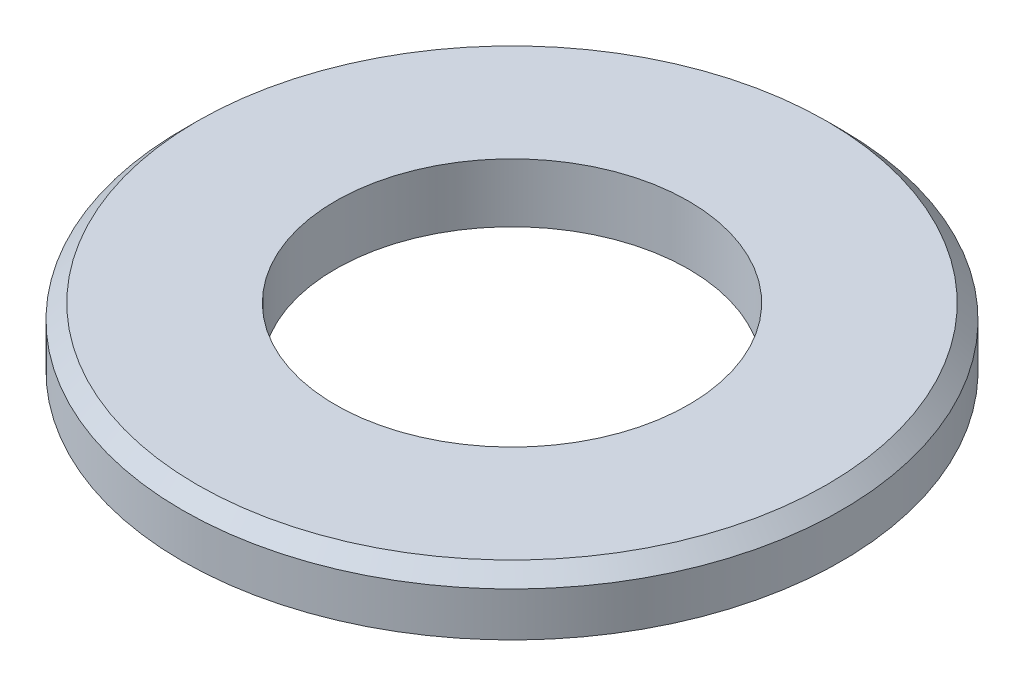
SolidWorks part; units mm, degrees
material "钢"
ref_plane "Plane1" through (0, 0, 0) normal (0, 0, 1) x (1, 0, 0)
ref_plane "Plane2" through (0, 0, 0) normal (0, 1, 0) x (1, 0, 0)
ref_plane "Plane3" through (0, 0, 0) normal (1, 0, 0) x (0, 0, -1)
sketch "Dimension sketch" plane through (0, 0, 0) normal (0, 0, 1) x (1, 0, 0)
  line L0 (0, 0) -> (9.1, 0)
  point P3 (2.5, 0)
  point P4 (28, 0)
  point P5 (15, 0)
sketch "Sketch1" plane through (0, 0, 0) normal (0, 0, 1) x (1, 0, 0)
  line L0 (0, 0) -> (0, 52.7318) construction
  line L1 (-13.375, 11.1445) -> (-14, 10.5195)
  line L2 (-7.5, 8.6445) -> (-14, 8.6445)
  line L3 (-7.5, 8.6445) -> (-7.5, 11.1445)
  line L4 (-7.5, 11.1445) -> (-13.375, 11.1445)
  line L5 (-14, 8.6445) -> (-14, 10.5195)
  point P4 (-14, 11.1445)
revolve "Base-Revolve" add sketch "Sketch1" angle 360 about L0
equation "\"h@Sketch1\" = \"h@Dimension sketch\""
equation "\"D1@Sketch1\" = \"d1@Dimension sketch\" / 2"
equation "\"D2@Sketch1\" = \"d2@Dimension sketch\" / 2"
equation "\"D5@Sketch1\" = \"h@Sketch1\" *0.25"
